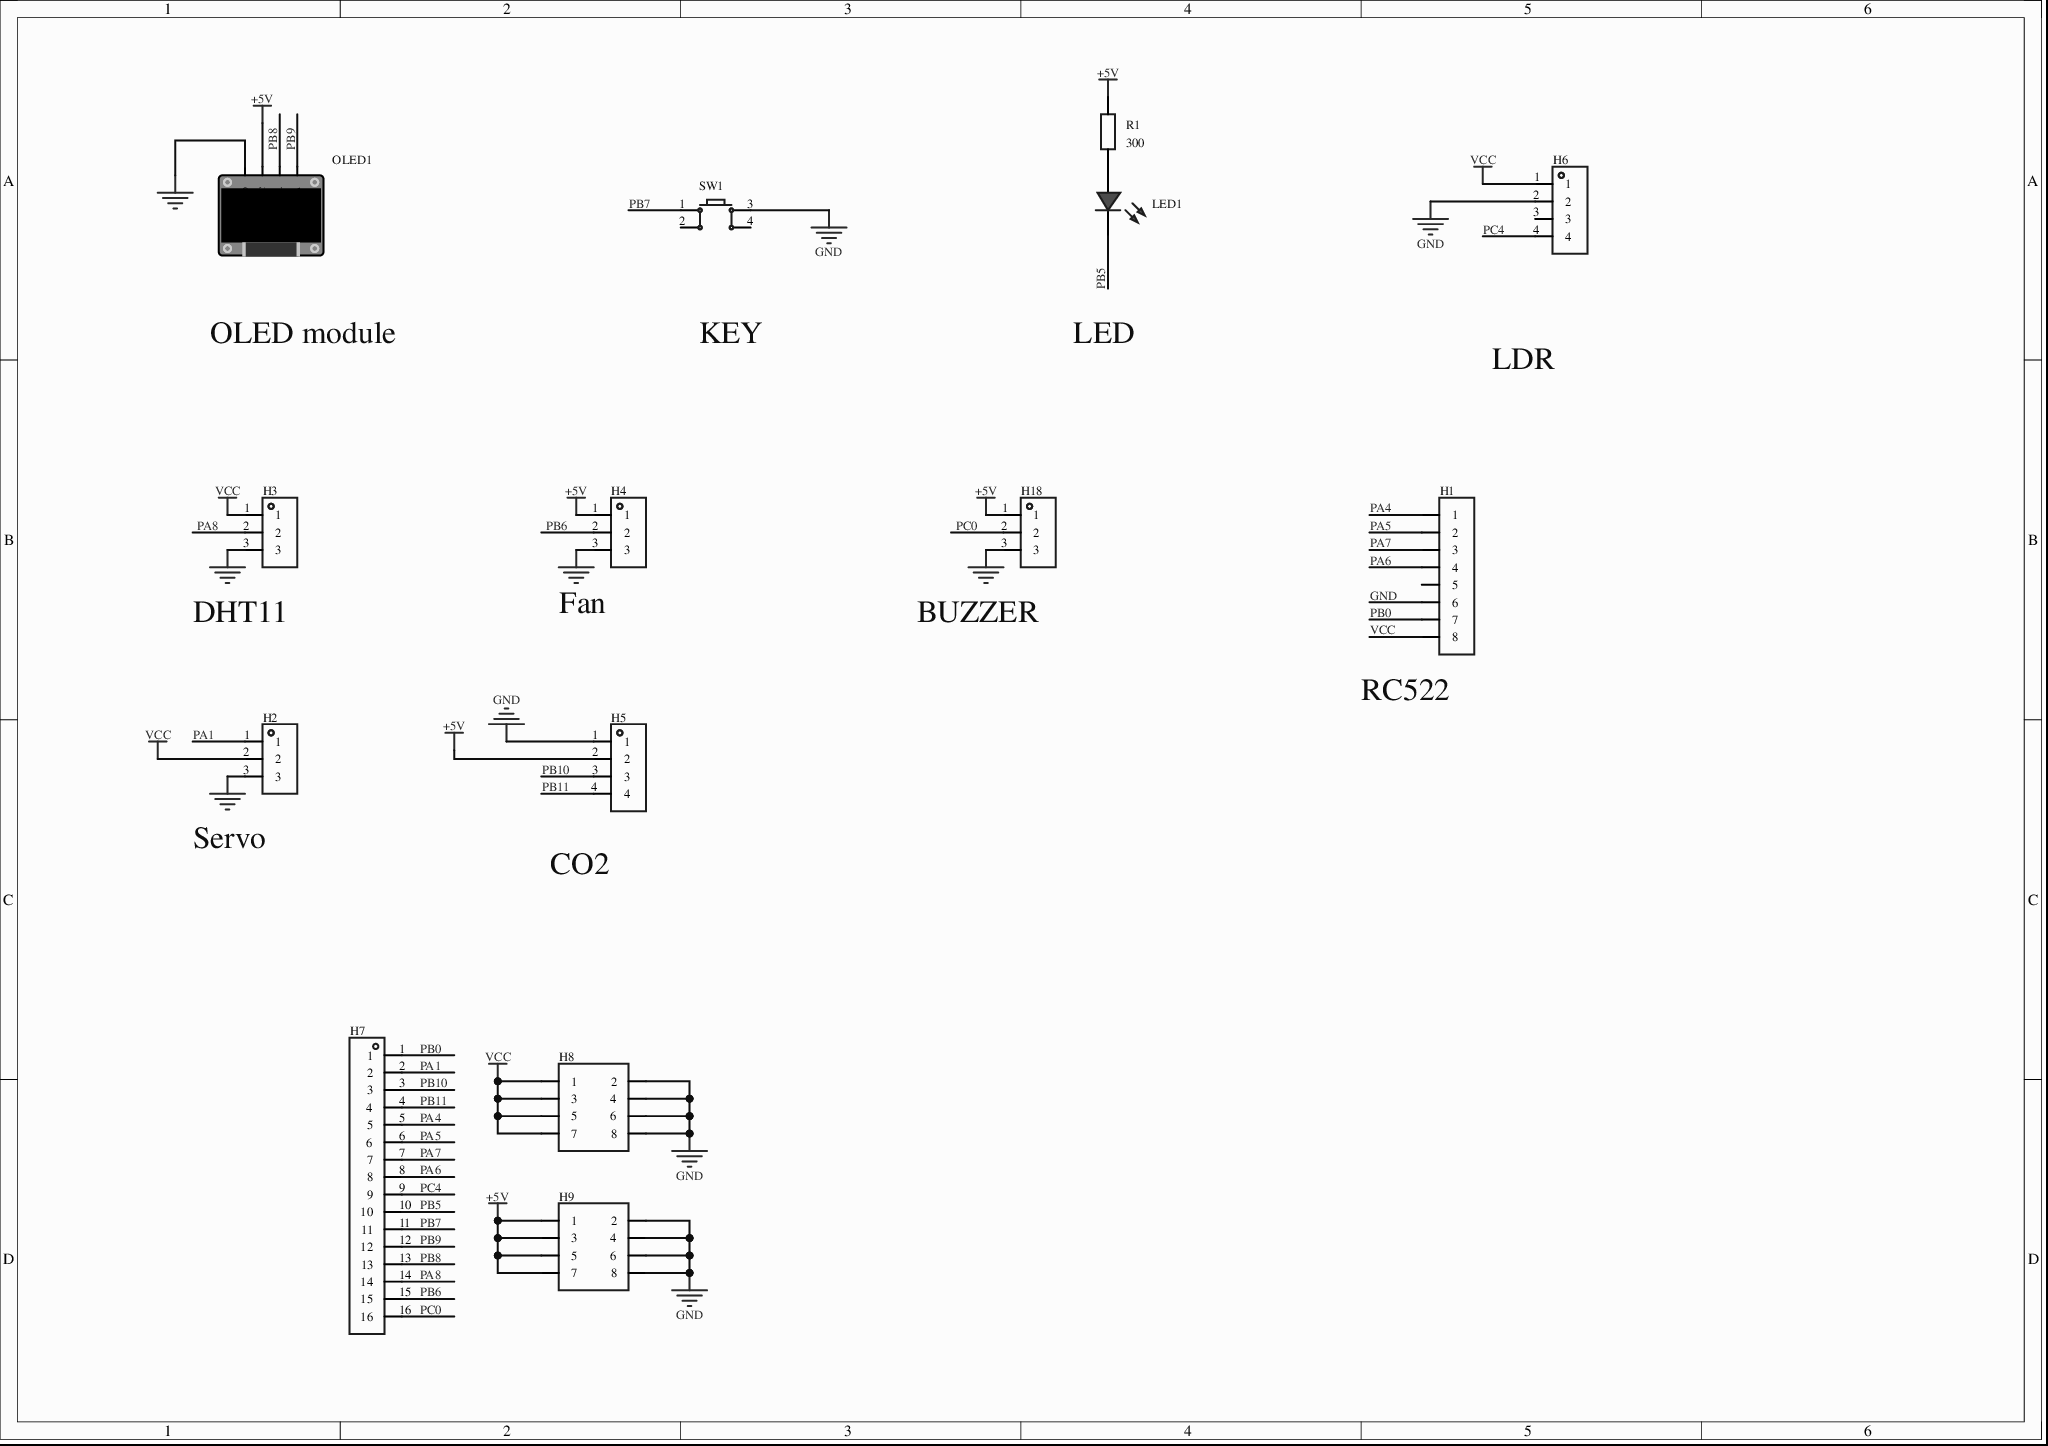
[diagram p0: MISC52124-3.schdoc]
# Altium project MISC52124-2.PrjPcb
1 sheet, 14 parts. Net scope: global (net labels, ports and power ports of the same name join across sheets).
Board file: MISC52124.pcbdoc

## Sheet MISC52124-3.schdoc
size 297 x 209 mm; Version: V1.0; @Project Name: MISC52124; @Page Count: 1; @Update Date: 2026-04-14; @Create Date: 2026-04-14; @Schematic Name: MISC52124; @Page No: 1; @Create Time: 23:22:16; @Update Time: 17:32:40; @Board Name: MISC52124

### Parts
H1  (no value)  [HDR-TH_8P-P2.54-V-F-1]
H2  (no value)  [HDR-TH_3P-P2.54-V-F]
H3  (no value)  [HDR-TH_3P-P2.54-V-F]
H4  (no value)  [HDR-TH_3P-P2.54-V-F]
H5  (no value)  [HDR-TH_4P-P2.54-V-F]
H6  (no value)  [HDR-TH_4P-P2.54-V-F]
H7  (no value)  [HDR-TH_16P-P2.54-V-F]
H8  (no value)  [HDR-TH_8P-P2.54-V-F-R2-C4-S2.54-1]
H9  (no value)  [HDR-TH_8P-P2.54-V-F-R2-C4-S2.54-1]
H18  (no value)  [HDR-TH_3P-P2.54-V-F]
LED1  (no value)  [LED_TH-3mm]
OLED1  (no value)  [0.96OLED_4P]
R1  300  [Res_1/8W]
SW1  (no value)  [SW-TH_4P-L6.0-W6.0-P4.50-LS6.5]

### Nets
+5V: H4.1 H5.2 H9.1 H9.3 H9.5 H9.7 H18.1 OLED1.2(VCC) R1.2
GND: H1.6 H2.3 H3.3 H4.3 H5.1 H6.2 H8.2 H8.4 H8.6 H8.8 H9.2 H9.4 H9.6 H9.8 H18.3 OLED1.1(GND) SW1.3
VCC: H1.8 H2.2 H3.1 H6.1 H8.1 H8.3 H8.5 H8.7
PA1: H2.1 H7.2
PA4: H1.1 H7.5
PA5: H1.2 H7.6
PA6: H1.4 H7.8
PA7: H1.3 H7.7
PA8: H3.2 H7.14
PB0: H1.7 H7.1
PB5: H7.10 LED1.2(A)
PB6: H4.2 H7.15
PB7: H7.11 SW1.1
PB8: H7.13 OLED1.3(SCL)
PB9: H7.12 OLED1.4(SDA)
PB10: H5.3 H7.3
PB11: H5.4 H7.4
PC0: H7.16 H18.2
PC4: H6.4 H7.9
NetLED1_1: LED1.1(C) R1.1

Not connected (* = marked no-connect by the designer): H1 5; H6 3; SW1 2 4

### Notes on the sheet
- OLED module
- KEY
- LED
- LDR
- (near H3) DHT11
- (near H4) Fan
- (near H18) BUZZER
- (near H1) RC522
- (near H2) Servo
- (near H5) CO2

### Library data of the parts
H1 = HDR-F_2.54_1x8P: Symbol: Header-Female-2.54_1x8; AddInBom: yes; ModelId: 0f7e4d9227ef4fa08d5469c22cc70cdb; ModelName: HDR-F-2.54_1x8; ModelTransform: 799.99844,100,0,0,0,0,0,0,-118.11; Device: HDR-F_2.54_1x8P; ConvertToPcb: yes; FootprintName: HDR-TH_8P-P2.54-V-F-1; SupplierPart: C27438; Supplier Footprint: 插件
H2-H4 = HDR-F_2.54_1x3P: Symbol: PM254V-11-03-H85; 3D Model: f3b3cc5aae9641bf9e56fc160cef875b; 3D Model Transform: 299.9994,100,0,0,0,0,0,0,-118.11; ConvertToPcb: yes; ModelName: HDR2.54-F-LI-1X3P; Device: HDR-F_2.54_1x3P; Supplier Part: C541850; Supplier Footprint: 插件; AddInBom: yes; FootprintName: HDR-TH_3P-P2.54-V-F
H5 H6 = HDR-F_2.54_1x4P: Symbol: 2.54-1*4P female; ConvertToPcb: yes; ModelId: d187812051054f85879fcaa51a310d8e0819f05c4eef4c71ace90d822a990e87; ModelTransform: 419.6842,98.464,0,0,0,0,0,0,-118.11; Device: HDR-F_2.54_1x4P; AddInBom: yes; SupplierPart: C2718488; Supplier Footprint: 插件; FootprintName: HDR-TH_4P-P2.54-V-F; ModelName: HDR-TH_4P-P2.54-V-F
H7 = HDR-F_2.54_1x16P: ConvertToPcb: yes; ModelId: 131891db3d2f4da4a154b1903ad8586e0819f05c4eef4c71ace90d822a990e87; ModelName: HDR-TH_16P-P2.54-F-LI-1X16P; ModelTransform: 1599.997,100,0,0,0,0,0,0,-118.11; Symbol: HDR-F_2.54_1x16P; Device: HDR-F_2.54_1x16P; AddInBom: yes; SupplierPart: C124409; Supplier Footprint: 插件; FootprintName: HDR-TH_16P-P2.54-V-F
H8 H9 = HDR-F_2.54_2x4: Symbol: HDR-F-2.54_2x4; ConvertToPcb: yes; ModelId: 64729f32a5874cf59655d275a66f10500819f05c4eef4c71ace90d822a990e87; ModelName: HDR2.54-F-LI-2X4P; ModelTransform: 399.999,200,0,0,0,0,0,0,-118.11; Device: HDR-F_2.54_2x4; AddInBom: yes; SupplierPart: C92271; Supplier Footprint: 插件; FootprintName: HDR-TH_8P-P2.54-V-F-R2-C4-S2.54-1
H18 = HDR-F_2.54_1x3P: Symbol: PM254V-11-03-H85; ConvertToPcb: yes; ModelId: f3b3cc5aae9641bf9e56fc160cef875b; ModelName: HDR2.54-F-LI-1X3P; ModelTransform: 299.9994,100,0,0,0,0,0,0,-118.11; Device: HDR-F_2.54_1x3P; AddInBom: yes; SupplierPart: C541850; Supplier Footprint: 插件; FootprintName: HDR-TH_3P-P2.54-V-F
LED1 = LED_TH-R_3mm: ConvertToPcb: yes; ModelId: a497c992633541038a38947cdc58012f0819f05c4eef4c71ace90d822a990e87; ModelName: LED-TH-3mm_R; ModelTransform: 141.274,153.327,0,0,0,0,-5.984,0,-137.795; Symbol: LED_TH-R; Device: LED_TH-R_3mm; AddInBom: yes; FootprintName: LED_TH-3mm; Supplier Footprint: 插件
OLED1 = 0.96OLED模块_4P: Device: 0.96OLED module_4P; ConvertToPcb: yes; ModelId: 79c000fdb68d45a296c2e9bedf4f9055; ModelTransform: 1393.69792,1318.895,0,0,0,0,0,-560.079,-137.795; Symbol: 0.96OLED module_4P; AddInBom: yes; FootprintName: 0.96OLED_4P; Supplier Footprint: 插件; ModelName: 0.96OLED_4P
R1 = Res_AXIAL-1/8W: Symbol: Resistor; 3D Model: b2b5ae7ae4c642178fe0039925c86a3f0819f05c4eef4c71ace90d822a990e87; 3D Model Transform: 282.86,66.88,253.09,0,0,0,0,0,-191; ConvertToPcb: yes; ModelName: RES-TH_BD1.8-L3.2-P7.20-D0.4; Device: Res_AXIAL-1/8W; Supplier Footprint: 轴向引线; Value: 300; AddInBom: yes; FootprintName: Res_1/8W
SW1 = Key_TH_6x6x6: Contact current:50mA;Rated voltage(DC):12V;Insulation resistance:100MΩ;Circuit structure:single pole single throw;Mounting:through-hole;Button shape:round button;Button/cap colour:black;Operating force:260gf@±30gf;Operating temperature:-25℃~+70℃;Pin style:PC pin;Switch length:6mm;Switch width:6mm;Switch height:6mm;With bracket:No;; Symbol: Tactile switch; 3D Model: 20eee248bc684ccd8cbdbb1d0d91ec6f; 3D Model Transform: 236.22,323.03,0,90,0,0,0,0,-137.795; ConvertToPcb: yes; ModelName: SW-TH_4P-L6.0-W6.0-H5.0-LS6.5-P4.50; Device: Key_TH_6x6x6; Supplier Part: C2837516; Supplier Footprint: 插件; AddInBom: yes; FootprintName: SW-TH_4P-L6.0-W6.0-P4.50-LS6.5